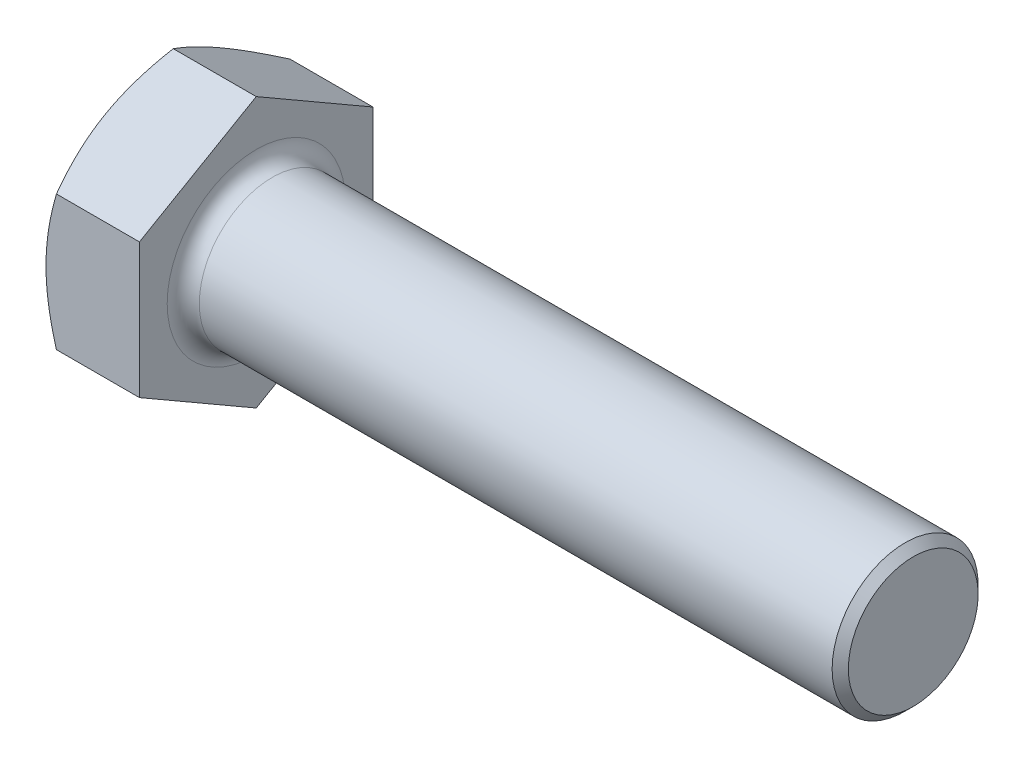
SolidWorks part; units mm, degrees
material "Q235"
ref_plane "Front Plane" through (0, 0, 0) normal (0, 0, 1) x (1, 0, 0)
ref_plane "Top Plane" through (0, 0, 0) normal (0, 1, 0) x (1, 0, 0)
ref_plane "Right Plane" through (0, 0, 0) normal (1, 0, 0) x (0, 0, -1)
sketch "Sketch1" plane through (0, 0, 0) normal (0, 0, 1) x (1, 0, 0)
  line L0 (0, 0) -> (51.4, 0) construction
  line L1 (0, 0) -> (0, 8.795)
  line L2 (0, 8.795) -> (6.4, 8.795)
  line L3 (6.4, 8.795) -> (6.4, 0)
  line L4 (6.4, 5) -> (51.4, 5)
  line L5 (51.4, 5) -> (51.4, 0)
  line L6 (0, 8) -> (0.459, 8.795)
  line L7 (48.4, 5) -> (48.4, 0)
  line L8 (10.9, 5) -> (10.9, 0)
  line L9 (6.4, 4.5129) -> (51.4, 4.5129)
  line L10 (51.4, 4.1881) -> (6.4, 4.1881)
  line L11 (5.8, 7.735) -> (6.4, 7.135)
  line L12 (5.8, 8.795) -> (5.8, 0)
  line L13 (6.3, 7.235) -> (6.3, 0) construction
  arc A0 (6.4, 6.1) -> (7.5, 5) centre (7.5, 6.1) ccw
  point P12 (49.9, 0)
  point P13 (2.23, 8.795)
  point P14 (6.4, 6.1)
  point P24 (6.4, 7.235)
  dimension "D1" = 0.1
  dimension "r" = 1.1
  dimension "k" = 6.4
  dimension "D2" = 45
  dimension "β" = 30
  dimension "e" = 17.59
  dimension "s" = 16
  dimension "d" = 10
  dimension "l" = 45
  dimension "D52" = 3
  dimension "P" = 1.5
  dimension "kw" = 4.17
  dimension "da" = 12.2
  dimension "a" = 4.5
  dimension "ds" = 9.0258
  dimension "D61" = 8.3763
  dimension "dw" = 14.47
  dimension "c" = 0.6
sketch "Sketch2" plane through (0, 0, 0) normal (1, 0, 0) x (0, 0, -1)
  line L1 (0, 9.2376) -> (-8, 4.6188)
  line L2 (-8, 4.6188) -> (-8, -4.6188)
  line L3 (-8, -4.6188) -> (0, -9.2376)
  line L4 (0, -9.2376) -> (8, -4.6188)
  line L5 (8, -4.6188) -> (8, 4.6188)
  line L6 (8, 4.6188) -> (0, 9.2376)
  circle A0 centre (0, 0) radius 8 construction
sketch "Sketch3" plane through (0, 0, 0) normal (1, 0, 0) x (0, 0, -1)
  line L0 (8, 4.6188) -> (0, 9.2376) construction
  line L1 (0, 9.2376) -> (-8, 4.6188) construction
  line L2 (-8, 4.6188) -> (-8, -4.6188) construction
  line L3 (8, -4.6188) -> (8, 4.6188) construction
  line L4 (0, -9.2376) -> (8, -4.6188) construction
  line L5 (-8, -4.6188) -> (0, -9.2376) construction
  line L6 (8, 4.6188) -> (0, 9.2376)
  line L7 (0, 9.2376) -> (-8, 4.6188)
  line L8 (-8, 4.6188) -> (-8, -4.6188)
  line L9 (8, -4.6188) -> (8, 4.6188)
  line L10 (0, -9.2376) -> (8, -4.6188)
  line L11 (-8, -4.6188) -> (0, -9.2376)
extrude "Boss-Extrude1" add sketch "Sketch3" along normal up to vertex (6.4 mm away) up to point (6.4, 8.795, 0)
sketch "Sketch4" plane through (0, 0, 0) normal (-1, 0, 0) x (0, 0, 1)
  circle A0 centre (0, 0) radius 8 construction
  circle A1 centre (0, 0) radius 8
  circle A2 centre (0, 0) radius 17.59
  dimension "D1" = 35.18
extrude "Cut-Extrude1" cut sketch "Sketch4" against normal blind 0.8 draft 60
sketch "Sketch5" plane through (0, 0, 0) normal (0, 0, 1) x (1, 0, 0)
  line L0 (6.4, 5) -> (51.4, 5) construction
  line L1 (51.4, 5) -> (51.4, 0) construction
  line L2 (0, 0) -> (51.4, 0) construction
  line L3 (7.5, 5) -> (51.4, 5)
  line L4 (51.4, 5) -> (51.4, 0)
  line L5 (6.4, 0) -> (51.4, 0)
  line L6 (6.4, 6.1) -> (6.4, 0)
  arc A0 (6.4, 6.1) -> (7.5, 5) centre (7.5, 6.1) ccw construction
  arc A1 (6.4, 6.1) -> (7.5, 5) centre (7.5, 6.1) ccw
revolve "Revolve1" add sketch "Sketch5" angle 360 about L5
cosmetic thread "Cosmetic Thread2" parameters "D1"=35.5, "D2"=8.3763
chamfer "Chamfer2" distance 0.5556 angle 45 1 edges at (51.4, 0, 5)
sketch "Sketch7" plane through (0, 0, 0) normal (0, 0, 1) x (1, 0, 0)
  line L0 (6.4, 7.135) -> (5.8, 7.735)
  line L1 (5.8, 7.735) -> (5.8, 17.59)
  line L2 (5.8, 17.59) -> (6.4, 17.59)
  line L3 (6.4, 17.59) -> (6.4, 7.135)
  line L4 (0, 0) -> (51.4, 0) construction
  line L5 (0, 0) -> (51.4, 0) construction
  dimension "D1" = 35.18
revolve "Cut-Revolve1" [suppressed] cut sketch "Sketch7" angle 360 mid plane about L5
sketch "Sketch6" [suppressed] plane through (0, 0, 0) normal (0, 0, 1) x (1, 0, 0)
  line L0 (5.9, 0) -> (5.9, 2.5) construction
  line L1 (5.9, 2.5) -> (13.5, 2.5)
  line L2 (13.5, 2.5) -> (13.5, 0)
  line L3 (5.9, 2.5) -> (4.069, 2.245)
  line L5 (3.5, 2.2402) -> (13.5, 2.2402) construction
  line L6 (3.5, 4.315) -> (3.5, 0) construction
  line L7 (3.5, 2.7402) -> (3.5, 0)
  line L8 (3.5, 0) -> (13.5, 0)
  arc A0 (4.069, 2.245) -> (3.5, 2.7402) centre (4, 2.7402) cw
  arc A1 (3.5, 3) -> (4, 2.5) centre (4, 3) ccw construction
revolve "Revolve2" add sketch "Sketch6" angle 360 about L8
cosmetic thread "Cosmetic Thread1" [suppressed] parameters "D1"=25.5, "D2"=8.3763
chamfer "Chamfer1" [suppressed] distance 0.5556 angle 45
sketch "Sketch8" plane through (0, 0, 0) normal (0, 0, 1) x (1, 0, 0)
  line L0 (6.4, 7.135) -> (5.8, 7.735)
  line L1 (5.8, 7.735) -> (5.8, 17.59)
  line L2 (5.8, 17.59) -> (6.4, 17.59)
  line L3 (6.4, 17.59) -> (6.4, 7.135)
  line L4 (0, 0) -> (51.4, 0) construction
  line L5 (0, 0) -> (51.4, 0) construction
  dimension "D1" = 35.18
revolve "Cut-Revolve2" [suppressed] cut sketch "Sketch8" angle 360 mid plane about L5
